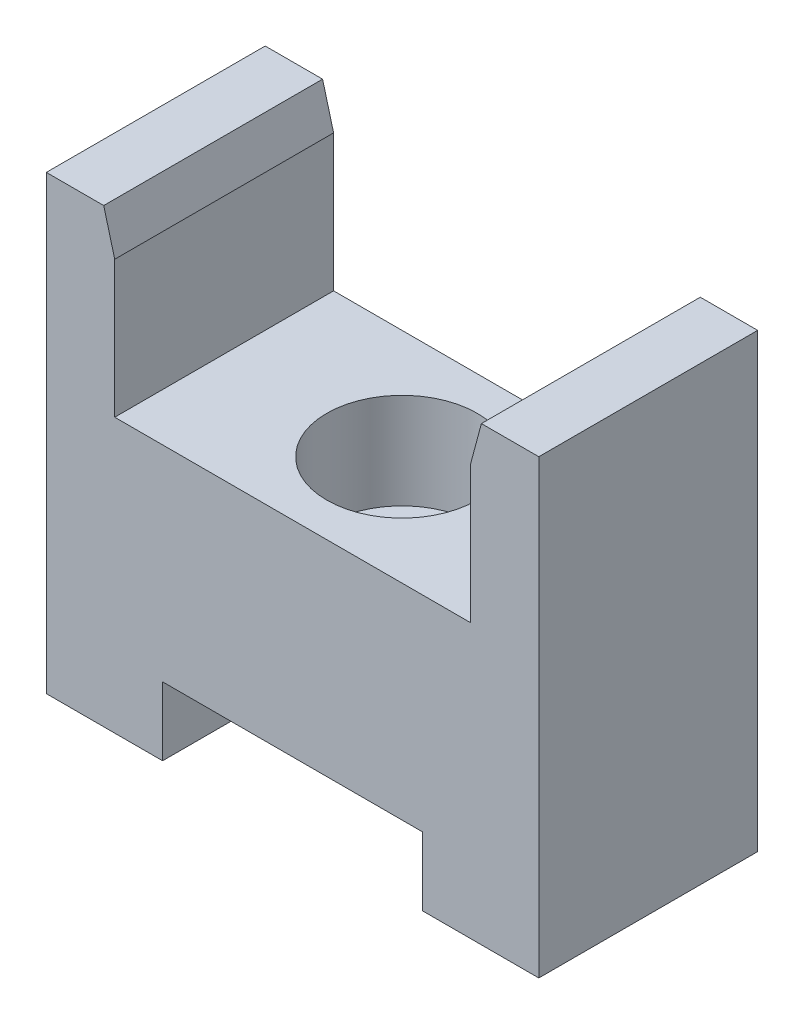
from build123d import *

# Parameters (mm, degrees)
BOSS_EXTRUDE1_DEPTH = 16
SKETCH2_R           = 5.5
CUT_EXTRUDE1_DEPTH  = 7
SKETCH3_R           = 3.5
CUT_EXTRUDE2_DEPTH  = 8


with BuildPart() as part:
    # Sketch1 → Boss-Extrude1 (new body)
    with BuildSketch(Plane.XY):
        Polygon((0, 33), (0, 0), (8.5, 0), (8.5, 5), (27.5, 5), (27.5, 0), (36, 0), (36, 33), (31.803847577, 33), (31, 30), (31, 20), (5, 20), (5, 30), (4.196152423, 33), align=None)
    extrude(amount=BOSS_EXTRUDE1_DEPTH)

    # Sketch2 → Cut-Extrude1 (cut)
    with BuildSketch(Plane(origin=(0, 20, 0), x_dir=(1, 0, 0), z_dir=(0, 1, 0))):
        with Locations(Location((18, -8, 0), (0, 0, 270))):
            Circle(SKETCH2_R)
    extrude(amount=-CUT_EXTRUDE1_DEPTH, mode=Mode.SUBTRACT)

    # Sketch3 → Cut-Extrude2 (cut)
    with BuildSketch(Plane(origin=(0, 13, 0), x_dir=(1, 0, 0), z_dir=(0, 1, 0))):
        with Locations(Location((18, -8, 0), (0, 0, 270))):
            Circle(SKETCH3_R)
    extrude(amount=-CUT_EXTRUDE2_DEPTH, mode=Mode.SUBTRACT)


solid = part.part
